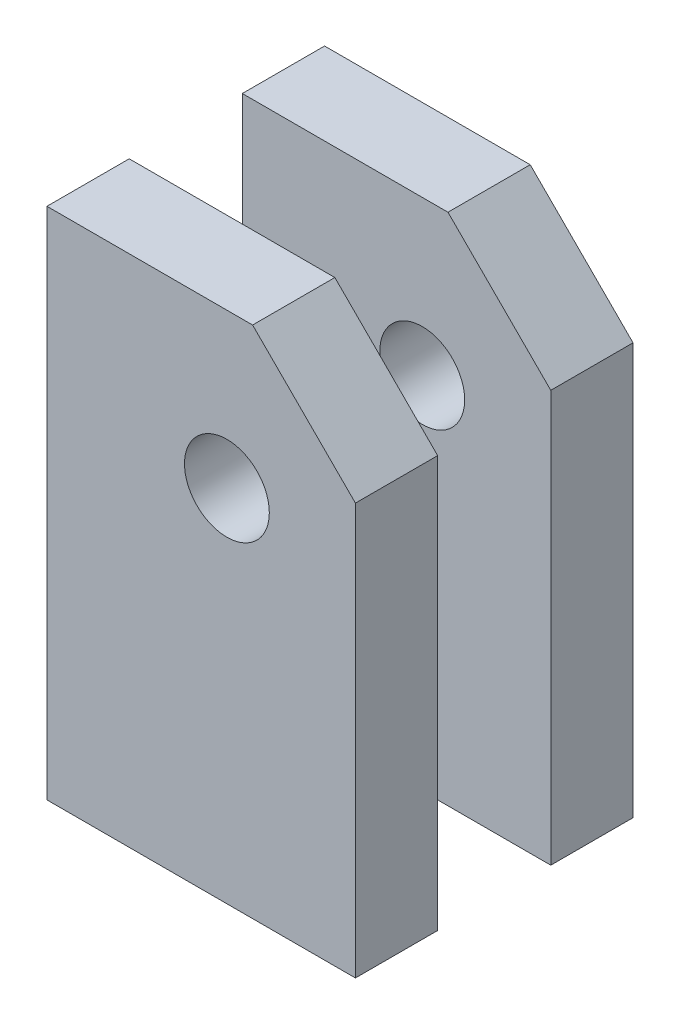
SolidWorks part; units mm, degrees
material "K"
ref_plane "Front" through (0, 0, 0) normal (0, 0, 1) x (1, 0, 0)
ref_plane "Top" through (0, 0, 0) normal (0, 1, 0) x (1, 0, 0)
ref_plane "Right" through (0, 0, 0) normal (1, 0, 0) x (0, 0, -1)
sketch "Sketch1" plane through (0, 0, 0) normal (0, 0, 1) x (1, 0, 0)
  line L1 (-30, -50) -> (30, -50)
  line L2 (-30, -50) -> (-30, 50)
  line L3 (-30, 50) -> (30, 50)
  line L4 (30, -50) -> (30, 50)
  line L5 (0, 50) -> (0, -50) construction
  line L6 (-30, 0) -> (30, 0) construction
  point P0 (0, 0)
  dimension "D1" = 60
  dimension "D2" = 100
extrude "Boss-Extrude1" add sketch "Sketch1" along normal blind 16
sketch "Sketch2" plane through (0, 0, 16) normal (0, 0, 1) x (1, 0, 0)
  line L0 (30, 50) -> (-30, 50) construction
  line L1 (-30, 50) -> (-30, -50) construction
  circle A0 centre (5, 20) radius 8.25
  dimension "D1" = 16.5
  dimension "D2" = 30
  dimension "D3" = 35
extrude "Cut-Extrude1" cut sketch "Sketch2" against normal blind 16
chamfer "Chamfer1" distance 20 angle 45 1 edges at (30, 50, 8)
ref_plane "Plane1" through (0, 0, -11) normal (0, 0, -1) x (-1, 0, 0)
mirror "Mirror1" about plane through (0, 0, -11) normal (0, 0, -1) of bodies 102
equation "\"零件重量\"= IIF ( \"SW-质量\" > 100 , int ( \"SW-质量\" ) , \"SW-质量\" )"
